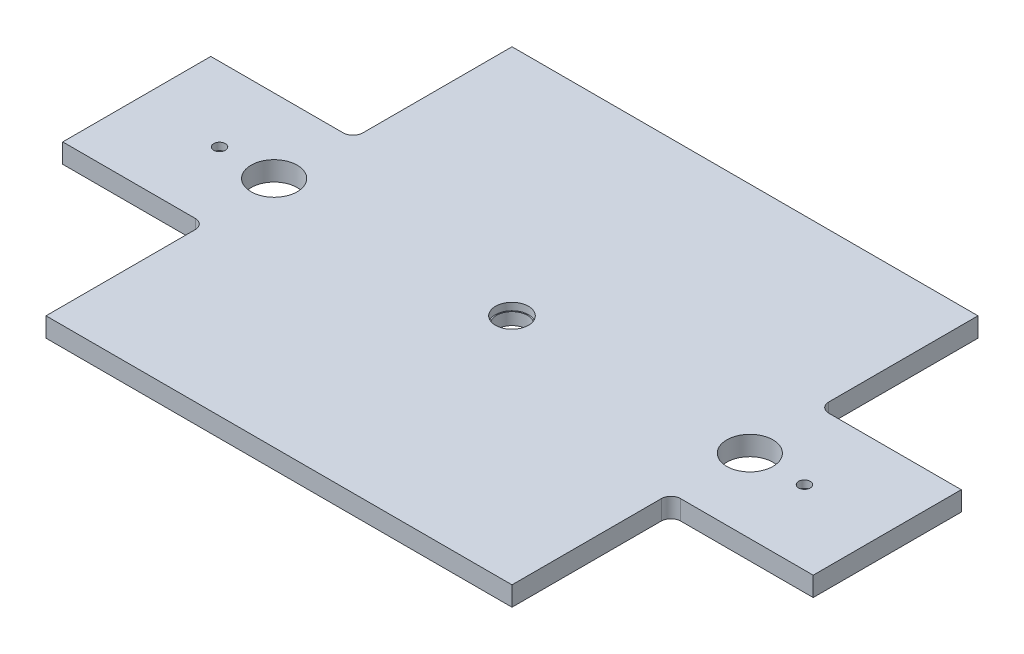
SolidWorks part; units mm, degrees
ref_plane "前视基准面" through (0, 0, 0) normal (0, 0, 1) x (1, 0, 0)
ref_plane "上视基准面" through (0, 0, 0) normal (0, 1, 0) x (1, 0, 0)
ref_plane "右视基准面" through (0, 0, 0) normal (1, 0, 0) x (0, 0, -1)
sketch "草图1" plane through (0, 0, 0) normal (0, 1, 0) x (1, 0, 0)
  line L0 (-480, 480) -> (480, 480)
  line L1 (480, 480) -> (480, 152.5)
  line L2 (480, 152.5) -> (773, 152.5)
  line L3 (773, 152.5) -> (773, -152.5)
  line L4 (773, -152.5) -> (480, -152.5)
  line L5 (480, -152.5) -> (480, -480)
  line L6 (480, -480) -> (-480, -480)
  line L7 (-480, -480) -> (-480, -152.5)
  line L8 (-480, -152.5) -> (-773, -152.5)
  line L9 (-773, -152.5) -> (-773, 152.5)
  line L10 (-773, 152.5) -> (-480, 152.5)
  line L11 (-480, 152.5) -> (-480, 480)
  line L12 (480, 480) -> (-480, -480) construction
  point P3 (0, 480)
  point P10 (0, 0)
  dimension "D1" = 960
  dimension "D2" = 960
  dimension "D3" = 305
  dimension "D4" = 293
extrude "凸台-拉伸1" add sketch "草图1" along normal blind 40
sketch "草图2" plane through (0, 0, 0) normal (0, -1, 0) x (1, 0, 0)
  line L0 (-773, -152.5) -> (-773, 152.5) construction
  line L1 (-773, 152.5) -> (-480, 152.5) construction
  circle A0 centre (602.5, 0) radius 20
  dimension "D1" = 40
  dimension "D2" = 1375.5
  dimension "D3" = 152.5
extrude "切除-拉伸1" cut sketch "草图2" against normal blind 10
hole_wizard "打孔尺寸(%根据)内六角圆柱头螺钉的类型0" positions "草图3" profile "草图4" counterbore size "M14" standard "GB" end condition through all
sketch "草图3" plane through (0, 40, 0) normal (0, 1, 0) x (1, 0, 0)
  line L0 (-480, -152.5) -> (-480, -480) construction
  line L1 (-480, -480) -> (480, -480) construction
  point P0 (602.5, 0)
  dimension "D1" = 1082.5
  dimension "D2" = 480
sketch "草图4" plane through (602.5, 40, 0) normal (1, 0, 0) x (0, 0, 1)
  line L0 (0, 0) -> (0, 40)
  line L1 (0, 40) -> (7.75, 40)
  line L3 (7.75, 40) -> (7.75, 15)
  line L4 (7.75, 15) -> (12, 15)
  line L5 (12, 15) -> (12, 0)
  line L7 (12, 0) -> (0, 0)
  line L11 (0, -6.35) -> (0, 107.95) construction
  dimension "通孔孔直径" = 15.5
  dimension "通孔孔深度" = 40
  dimension "柱形沉头孔直径" = 24
  dimension "柱形沉头孔深度" = 15
mirror "镜向1" about plane through (0, 0, 0) normal (1, 0, 0) of "切除-拉伸1", "打孔尺寸(%根据)内六角圆柱头螺钉的类型0"
sketch "草图5" plane through (0, 0, 0) normal (0, -1, 0) x (1, 0, 0)
  line L0 (-773, -152.5) -> (-773, 152.5) construction
  line L1 (-773, 152.5) -> (-480, 152.5) construction
  circle A0 centre (490, 0) radius 47.5
  dimension "D1" = 95
  dimension "D2" = 1263
  dimension "D3" = 152.5
extrude "切除-拉伸2" cut sketch "草图5" against normal through all
mirror "镜向2" about plane through (0, 0, 0) normal (1, 0, 0) of "切除-拉伸2"
sketch "草图6" plane through (0, 40, 0) normal (0, 1, 0) x (1, 0, 0)
  line L0 (-480, -152.5) -> (-480, -480) construction
  line L1 (-480, -480) -> (480, -480) construction
  circle A0 centre (0, 0) radius 31.75
  dimension "D1" = 63.5
  dimension "D2" = 480
  dimension "D3" = 480
extrude "切除-拉伸3" cut sketch "草图6" against normal through all
fillet "圆角1" radius 20 4 edges at (-480, 20, 152.5) (-480, 20, -152.5) (480, 20, 152.5) (480, 20, -152.5)
sketch "草图7" plane through (0, 40, 0) normal (0, 1, 0) x (1, 0, 0)
  line L0 (480, -480) -> (480, -172.5) construction
  line L1 (-480, -480) -> (480, -480) construction
  circle A0 centre (0, 0) radius 34
  dimension "D1" = 68
  dimension "D2" = 480
  dimension "D3" = 480
extrude "切除-拉伸4" cut sketch "草图7" against normal blind 15
